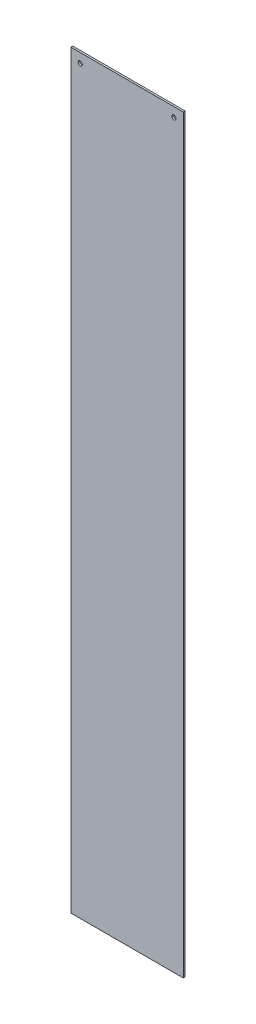
SolidWorks part; units mm, degrees
material "PVC 0.007 塑化"
ref_plane "前视基准面" through (0, 0, 0) normal (0, 0, 1) x (1, 0, 0)
ref_plane "上视基准面" through (0, 0, 0) normal (0, 1, 0) x (1, 0, 0)
ref_plane "右视基准面" through (0, 0, 0) normal (1, 0, 0) x (0, 0, -1)
sketch "草图1" plane through (0, 0, 0) normal (0, 0, 1) x (1, 0, 0)
  line L1 (-60, 400) -> (60, 400)
  line L2 (-60, 400) -> (-60, -400)
  line L3 (-60, -400) -> (60, -400)
  line L4 (60, 400) -> (60, -400)
  line L5 (0, -400) -> (0, 400) construction
  line L6 (-60, 0) -> (60, 0) construction
  point P0 (0, 0)
  dimension "D1" = 120
  dimension "D2" = 800
extrude "凸台-拉伸1" add sketch "草图1" along normal blind 2
sketch "草图2" plane through (0, 0, 2) normal (0, 0, 1) x (1, 0, 0)
  line L0 (0, 400) -> (0, -400) construction
  line L1 (60, 400) -> (-60, 400) construction
  line L2 (-60, -400) -> (60, -400) construction
  line L3 (-50, 390) -> (50, 390) construction
  circle A0 centre (-50, 390) radius 2.25
  circle A1 centre (50, 390) radius 2.25
  dimension "D3" = 4.5
  dimension "D1" = 100
  dimension "D2" = 10
extrude "切除-拉伸1" cut sketch "草图2" against normal blind 10
